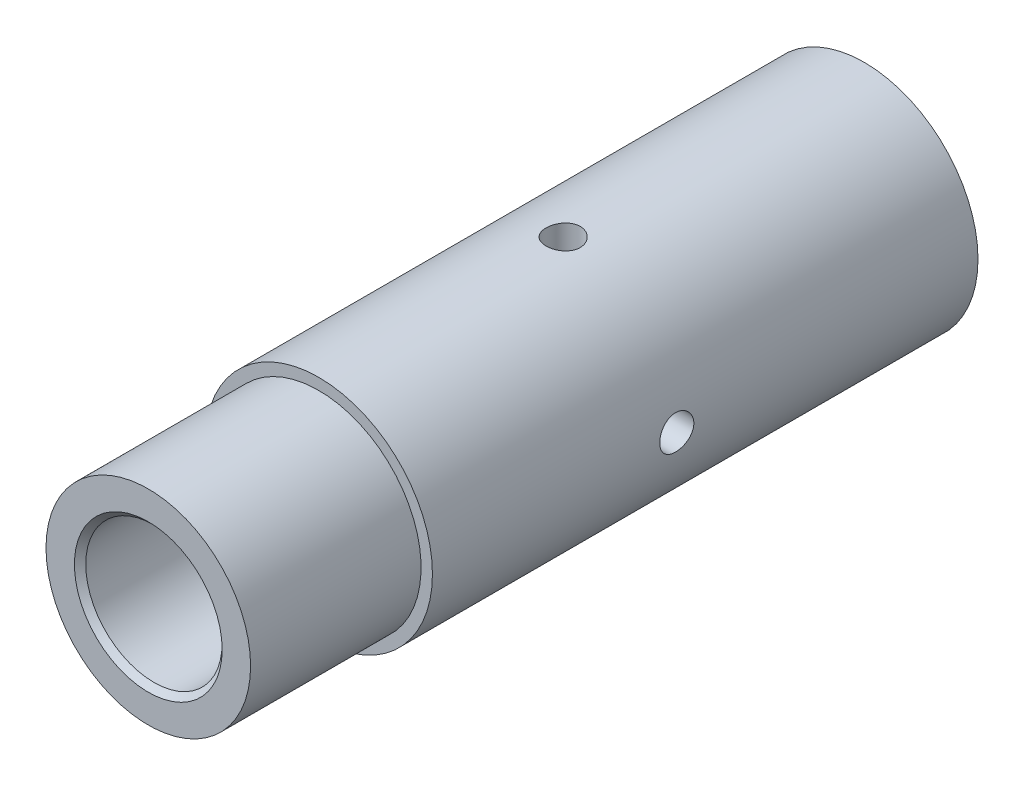
from build123d import *

# Parameters (mm, degrees)
SKETCH1_R           = 9
BOSS_EXTRUDE1_DEPTH = 63
SKETCH2_R           = 10
BOSS_EXTRUDE2_DEPTH = 48
SKETCH3_R           = 6
CUT_EXTRUDE1_DEPTH  = 65.567793829
SKETCH4_W           = 1.5
SKETCH4_H           = 27.68
CIRPATTERN1_COUNT   = 4
CHAMFER1_SIZE       = 0.5


with BuildPart() as part:
    # Sketch1 → Boss-Extrude1 (new body)
    with BuildSketch(Plane.XY):
        Circle(SKETCH1_R)
    extrude(amount=BOSS_EXTRUDE1_DEPTH)

    # Sketch2 → Boss-Extrude2 (add)
    with BuildSketch(Plane(origin=(0, 0, 0), x_dir=(-1, 0, 0), z_dir=(0, 0, -1))):
        Circle(SKETCH2_R)
    extrude(amount=-BOSS_EXTRUDE2_DEPTH)

    # Sketch3 → Cut-Extrude1 (cut, through all)
    with BuildSketch(Plane(origin=(0, 0, 0), x_dir=(-1, 0, 0), z_dir=(0, 0, -1))):
        Circle(SKETCH3_R)
    extrude(amount=-CUT_EXTRUDE1_DEPTH, mode=Mode.SUBTRACT)

    # Sketch4 → Cut-Revolve1 (revolve, cut)
    with BuildSketch(Plane(origin=(0, 0, 0), x_dir=(0, 0, -1), z_dir=(1, 0, 0)), mode=Mode.PRIVATE) as cut_revolve1_sk:
        with Locations((-25.75, 0.585439351)):
            Rectangle(SKETCH4_W, SKETCH4_H)
    cut_revolve1 = revolve(cut_revolve1_sk.sketch.rotate(Axis((0, 14.425439351, 26.5), (0, -1, 0)), 180), axis=Axis((0, 14.425439351, 26.5), (0, -1, 0)), mode=Mode.SUBTRACT)

    # CirPattern1: Cut-Revolve1 ×4 about axis
    cirpattern1_axis = Axis((0, 0, 48), (0, 0, -1))
    for i in range(1, CIRPATTERN1_COUNT):
        add(cut_revolve1.rotate(cirpattern1_axis, i * 360 / CIRPATTERN1_COUNT), mode=Mode.SUBTRACT)

    # Chamfer1
    chamfer1_edges = [part.edges().sort_by_distance(p)[0] for p in [
        (6, 0, 63),
    ]]
    chamfer(chamfer1_edges, length=CHAMFER1_SIZE)


solid = part.part
